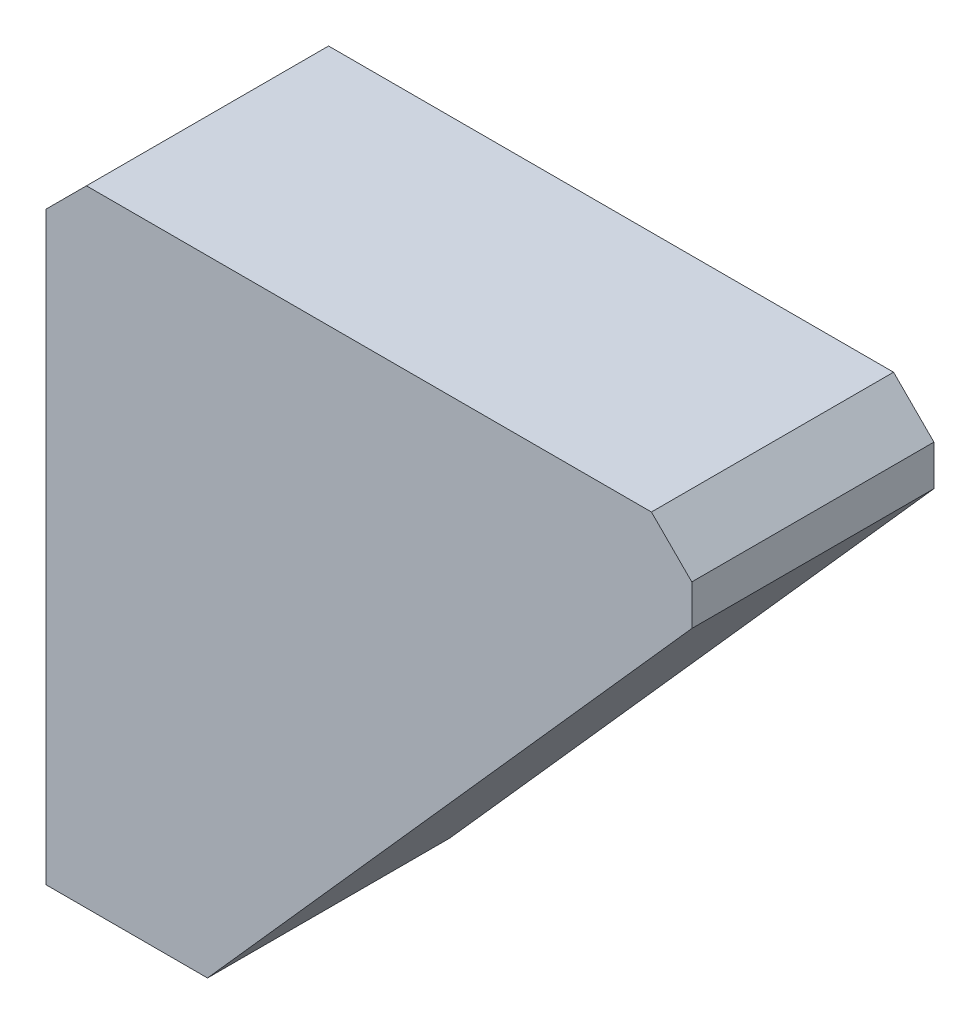
from build123d import *

# Parameters (mm, degrees)
BOSS_EXTRUDE1_DEPTH = 30


with BuildPart() as part:
    # Sketch1 → Boss-Extrude1 (new body)
    with BuildSketch(Plane.XY):
        Polygon((0, 0), (0, 72.5), (5, 77.5), (75, 77.5), (80, 72.5), (80, 67.5), (20, 0), align=None)
    extrude(amount=BOSS_EXTRUDE1_DEPTH)


solid = part.part
